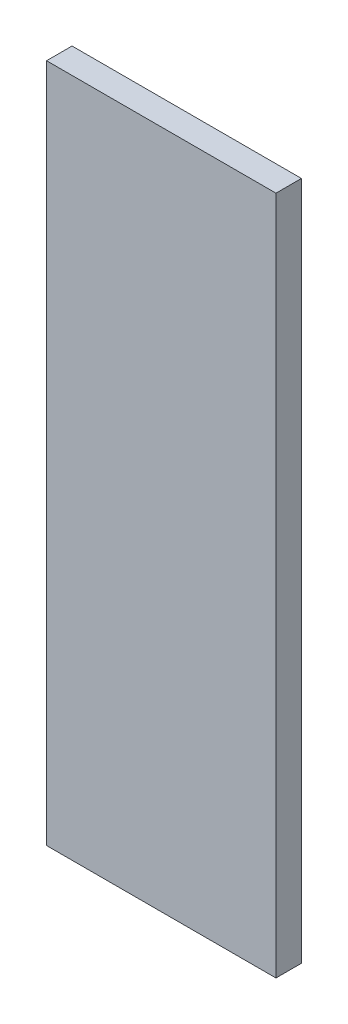
from build123d import *

# Parameters (mm, degrees)
SKETCH_1_W          = 27
SKETCH_1_H          = 80
EXTRUDE_2_DEPTH     = 3
SKETCH_2_R          = 1
CUT_EXTRUDE_1_DEPTH = 15


with BuildPart() as part:
    # 草图1 → 凸台-拉伸2 (new body)
    with BuildSketch(Plane.XY):
        with Locations((-21.456521739, -18.02173913)):
            Rectangle(SKETCH_1_W, SKETCH_1_H)
    extrude(amount=EXTRUDE_2_DEPTH)

    # 草图2 → 切除-拉伸1 (cut)
    with BuildSketch(Plane(origin=(820.104098161, -68.02173913, 1111.231170435), x_dir=(-0.9925461516413246, -2.2389179114641602e-14, -0.12186934340512692), z_dir=(0, -1, 0))):
        with Locations(Location((963.085867609, 999.8129825, 0), (0, 0, 83))):
            Circle(SKETCH_2_R)
        with Locations(Location((977.974059883, 997.984942349, 0), (0, 0, 83))):
            Circle(SKETCH_2_R)
        with Locations((961.501566145, 986.909882529)):
            Circle(SKETCH_2_R)
        with Locations((976.389758419, 985.081842378)):
            Circle(SKETCH_2_R)
    extrude(amount=-CUT_EXTRUDE_1_DEPTH, mode=Mode.SUBTRACT)


solid = part.part
